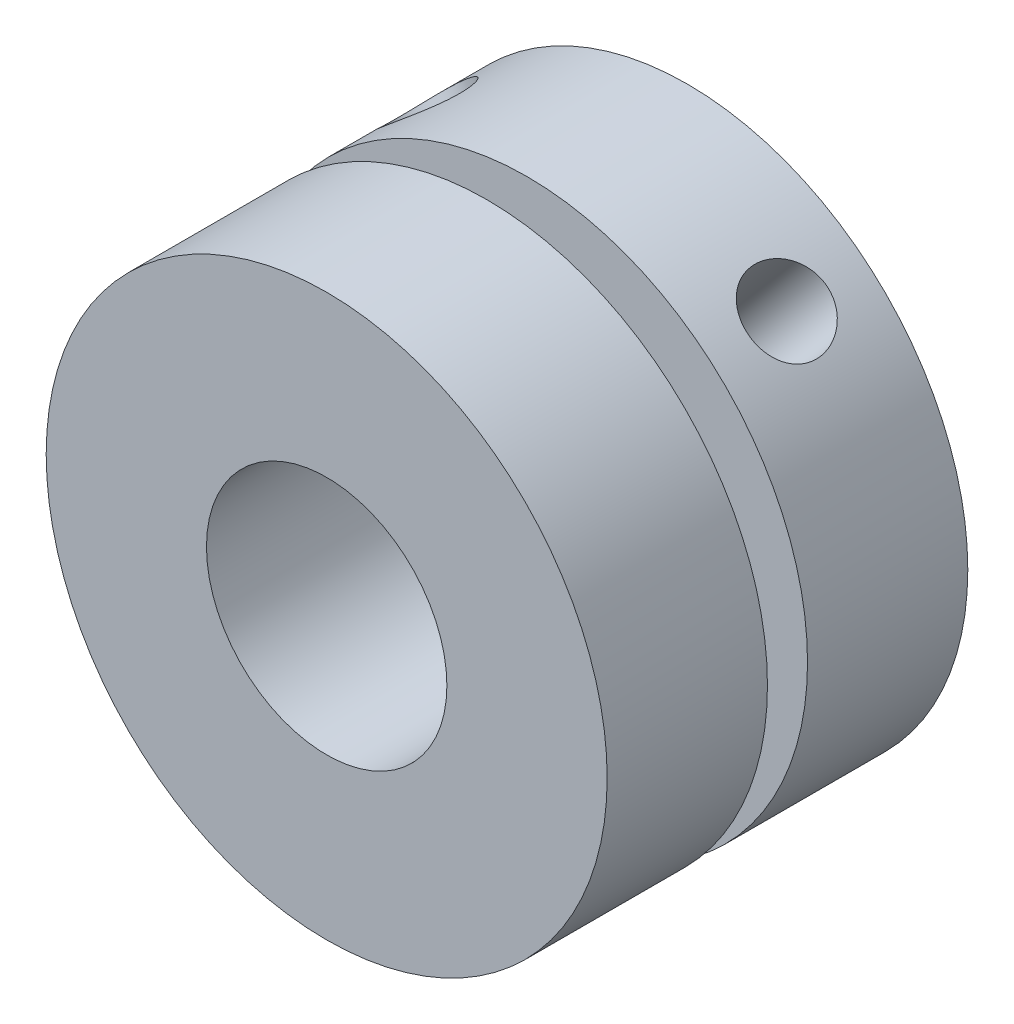
SolidWorks part; units mm, degrees
ref_plane "Front Plane" through (0, 0, 0) normal (0, 0, 1) x (1, 0, 0)
ref_plane "Top Plane" through (0, 0, 0) normal (0, 1, 0) x (1, 0, 0)
ref_plane "Right Plane" through (0, 0, 0) normal (1, 0, 0) x (0, 0, -1)
other "Configuration Table"
sketch "Sketch1" plane through (0, 0, 0) normal (0, 0, 1) x (1, 0, 0)
  circle A0 centre (0, 0) radius 35
  circle A1 centre (0, 0) radius 15
  dimension "D1" = 70
  dimension "D2" = 30
extrude "Boss-Extrude1" add sketch "Sketch1" along normal blind 20 contours A0 | A1
sketch "Sketch2" plane through (0, 0, 0) normal (0, 0, -1) x (-1, 0, 0)
  circle A0 centre (0, 0) radius 15 construction
  circle A1 centre (0, 0) radius 35
  circle A2 centre (0, 0) radius 35
  circle A3 centre (0, 0) radius 15
  circle A4 centre (0, 0) radius 20
  circle M5 centre (0, 0) radius 15
  dimension "D2" = 40
  dimension "D1" = 0
extrude "Boss-Extrude2" add sketch "Sketch2" along normal mid plane 10 contours A4 M5
sketch "Sketch5" plane through (0, 0, -5) normal (0, 0, -1) x (-1, 0, 0)
  circle A0 centre (0, 0) radius 35
  circle A1 centre (0, 0) radius 15 construction
  circle A2 centre (0, 0) radius 15
extrude "Boss-Extrude3" add sketch "Sketch5" along normal blind 20 contours A0
sketch "Sketch6" plane through (0, 0, -25) normal (0, 0, -1) x (-1, 0, 0)
  circle A0 centre (0, 0) radius 20
  dimension "D1" = 40
extrude "Boss-Extrude4" add sketch "Sketch6" along normal blind 10
ref_plane "Plane3" through (0, 0, -15) normal (0, 0, 1) x (1, 0, 0)
sketch "Sketch11" plane through (0, 0, -15) normal (0, 0, 1) x (1, 0, 0)
  line L0 (0, 36.5285) -> (0, 0) construction
  line L1 (-11.6234, 13.8523) -> (-23.2468, 27.7045)
  line L2 (-23.2468, 27.7045) -> (-19.4166, 30.9184)
  line L3 (-19.4166, 30.9184) -> (-7.7932, 17.0662)
  line L4 (-7.7932, 17.0662) -> (-11.6234, 13.8523)
  dimension "D1" = 40
  dimension "D2" = 5
revolve "Cut-Revolve2" cut sketch "Sketch11" angle 360 about L1
cosmetic thread "Cosmetic Thread1" parameters "D2"=12
sketch "Sketch17" plane through (0, 0, -15) normal (0, 0, 1) x (1, 0, 0)
  line L0 (0, 0) -> (0, 37.2486) construction
  line L1 (12.4508, 14.8383) -> (24.4167, 29.0986)
  line L2 (24.4167, 29.0986) -> (28.2469, 25.8847)
  line L3 (28.2469, 25.8847) -> (16.281, 11.6244)
  line L4 (16.281, 11.6244) -> (12.4508, 14.8383)
  dimension "D1" = 5
  dimension "D2" = 40
revolve "Cut-Revolve3" cut sketch "Sketch17" angle 360 about L1
cosmetic thread "Cosmetic Thread2" parameters "D2"=12
